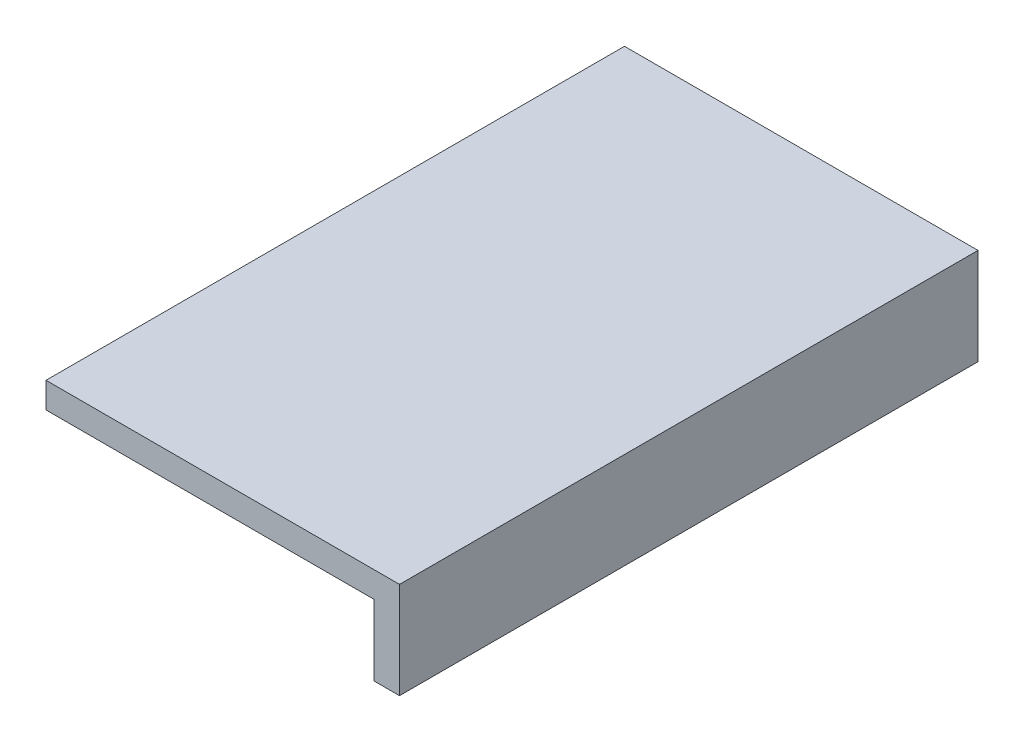
from build123d import *

# Parameters (mm, degrees)
EXTRUDE_1_DEPTH = 180


with BuildPart() as part:
    # 草图1 → 凸台-拉伸1 (new body)
    with BuildSketch(Plane.XY):
        Polygon((0, 0), (110, 0), (110, -30), (102, -30), (102, -8), (0, -8), align=None)
    extrude(amount=EXTRUDE_1_DEPTH)


solid = part.part
